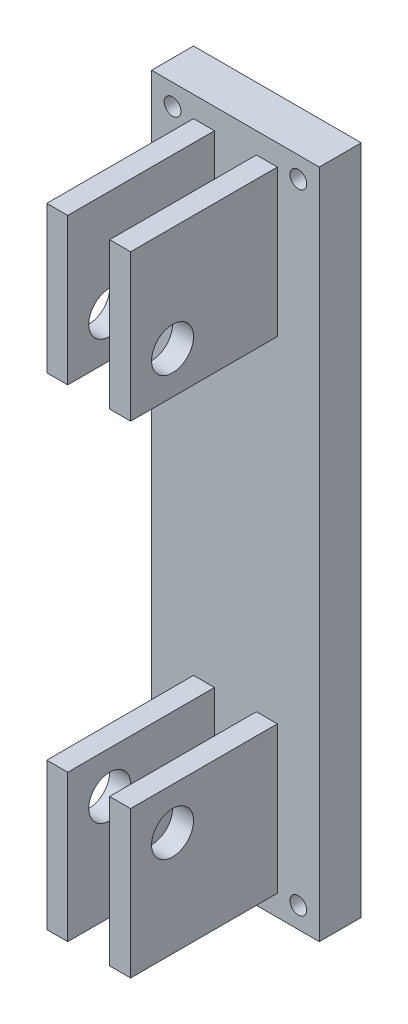
from build123d import *

# Parameters (mm, degrees)
SKETCH1_W           = 4
SKETCH1_H           = 16
BOSS_EXTRUDE1_DEPTH = 1
SKETCH2_W           = 0.5
SKETCH2_H           = 15
BOSS_EXTRUDE2_DEPTH = 3.5
SKETCH3_R           = 0.5
CUT_EXTRUDE1_DEPTH  = 4.5
SKETCH4_R           = 0.2
CUT_EXTRUDE2_DEPTH  = 4.5
SKETCH5_W           = 8.19252636
SKETCH5_H           = 8
CUT_EXTRUDE3_DEPTH  = 3.5


with BuildPart() as part:
    # Sketch1 → Boss-Extrude1 (new body)
    with BuildSketch(Plane.XY):
        Rectangle(SKETCH1_W, SKETCH1_H)
    extrude(amount=BOSS_EXTRUDE1_DEPTH)

    # Sketch2 → Boss-Extrude2 (add)
    with BuildSketch(Plane.XY.offset(1)):
        with Locations((0.75, 0)):
            Rectangle(SKETCH2_W, SKETCH2_H)
        with Locations((-0.75, 0)):
            Rectangle(SKETCH2_W, SKETCH2_H)
    extrude(amount=BOSS_EXTRUDE2_DEPTH)

    # Sketch3 → Cut-Extrude1 (cut)
    with BuildSketch(Plane.ZY.offset(1)):
        with Locations((3.5, 5)):
            Circle(SKETCH3_R)
        with Locations((3.5, -5)):
            Circle(SKETCH3_R)
    extrude(amount=-CUT_EXTRUDE1_DEPTH, mode=Mode.SUBTRACT)

    # Sketch4 → Cut-Extrude2 (cut)
    with BuildSketch(Plane.XY.offset(1)):
        with Locations((-1.5, 7.5)):
            Circle(SKETCH4_R)
        with Locations((-1.5, -7.5)):
            Circle(SKETCH4_R)
        with Locations((1.5, -7.5)):
            Circle(SKETCH4_R)
        with Locations((1.5, 7.5)):
            Circle(SKETCH4_R)
    extrude(amount=-CUT_EXTRUDE2_DEPTH, mode=Mode.SUBTRACT)

    # Sketch5 → Cut-Extrude3 (cut)
    with BuildSketch(Plane.XY.offset(4.5)):
        Rectangle(SKETCH5_W, SKETCH5_H)
    extrude(amount=-CUT_EXTRUDE3_DEPTH, mode=Mode.SUBTRACT)


solid = part.part
